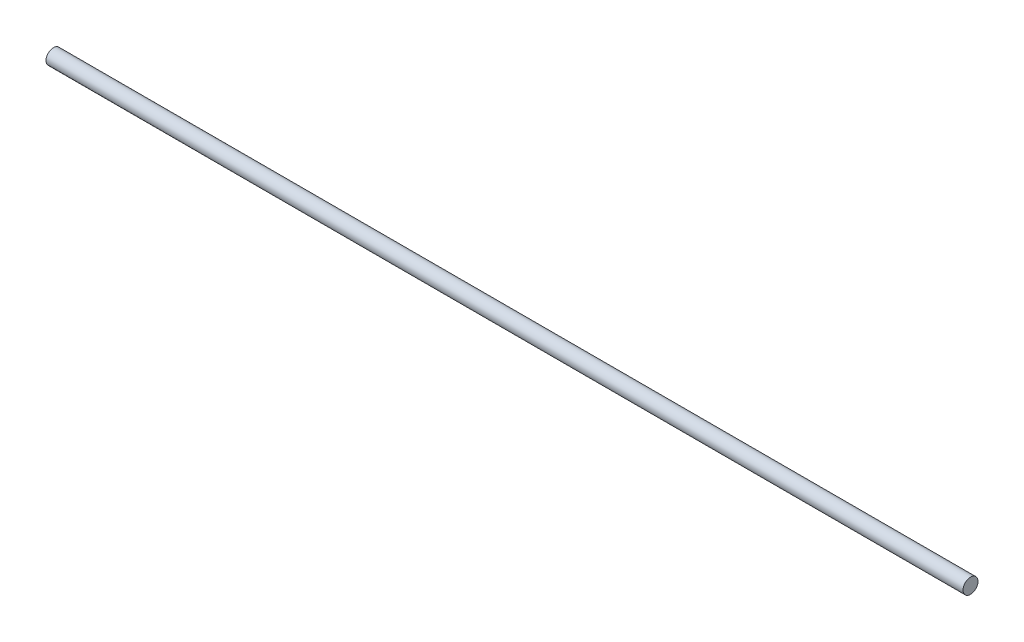
from build123d import *

# Parameters (mm, degrees)
SKETCH1_W = 767
SKETCH1_H = 12.5


with BuildPart() as part:
    # Sketch1 → Revolve1 (revolve)
    with BuildSketch(Plane.XY, mode=Mode.PRIVATE) as revolve1_sk:
        with Locations((-383.5, 6.25)):
            Rectangle(SKETCH1_W, SKETCH1_H)
    revolve1 = revolve(revolve1_sk.sketch.rotate(Axis((-202.604499093, 0, 0), (1, 0, 0)), 90), axis=Axis((-202.604499093, 0, 0), (1, 0, 0)))

    # Mirror1: Revolve1 across plane
    add(revolve1.mirror(Plane(origin=(0, 0, 0), x_dir=(0, 0, 1), z_dir=(1, 0, 0))))


solid = part.part
